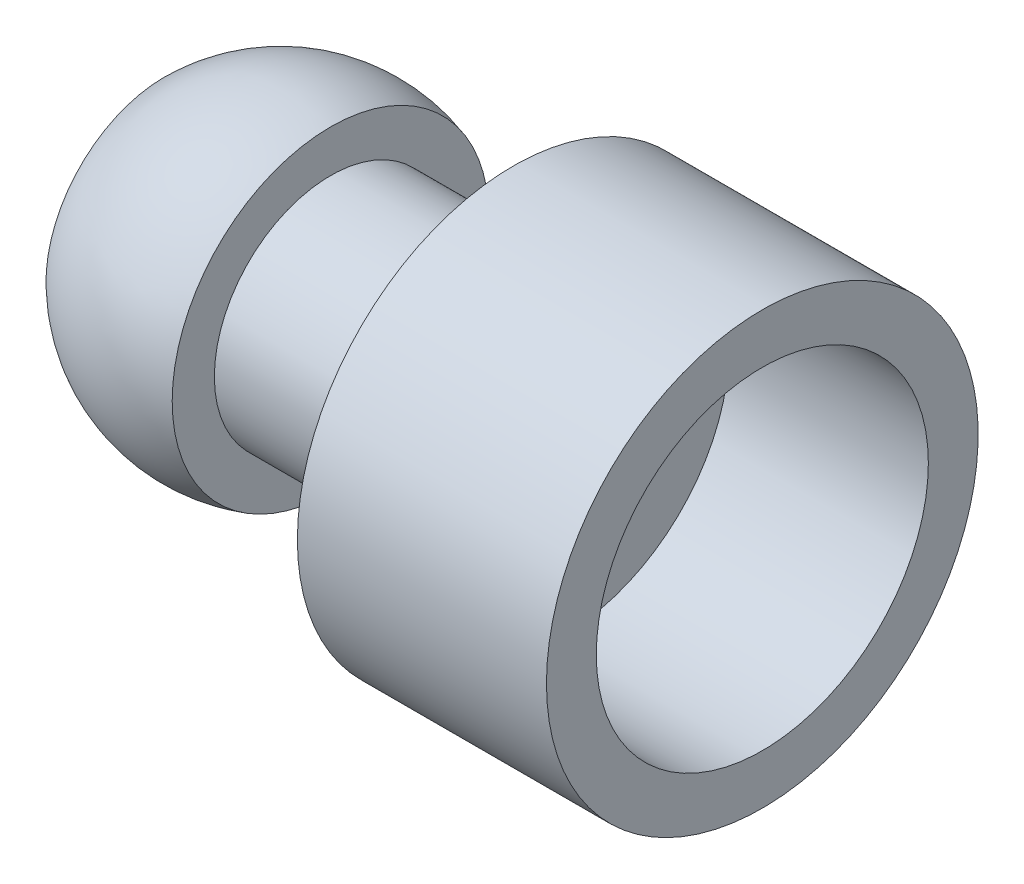
SolidWorks part; units mm, degrees
ref_plane "Front Plane" through (0, 0, 0) normal (0, 0, 1) x (1, 0, 0)
ref_plane "Top Plane" through (0, 0, 0) normal (0, 1, 0) x (1, 0, 0)
ref_plane "Right Plane" through (0, 0, 0) normal (1, 0, 0) x (0, 0, -1)
other "Configuration Table"
ref_plane "Plane1" through (0, 0, 0) normal (0, 0, -1) x (-1, 0, 0)
sketch "Sketch1" plane through (0, 0, 0) normal (0, 0, -1) x (-1, 0, 0)
  line L0 (21, 5) -> (23.8868, 0)
  line L1 (23.8868, 0) -> (36, 0)
  line L2 (36, 0) -> (36, 7.1414)
  line L3 (26, 9.5394) -> (26, 7)
  line L4 (26, 7) -> (15, 7)
  line L5 (15, 7) -> (15, 13)
  line L6 (15, 13) -> (0, 13)
  line L7 (0, 13) -> (0, 10)
  line L8 (0, 10) -> (12, 10)
  line L9 (12, 10) -> (12, 5)
  line L10 (12, 5) -> (21, 5)
  line L11 (0, 0) -> (36, 0) construction
  arc A0 (36, 7.1414) -> (26, 9.5394) centre (29, 0) ccw
revolve "Revolve1" add sketch "Sketch1" angle 360 about L11
